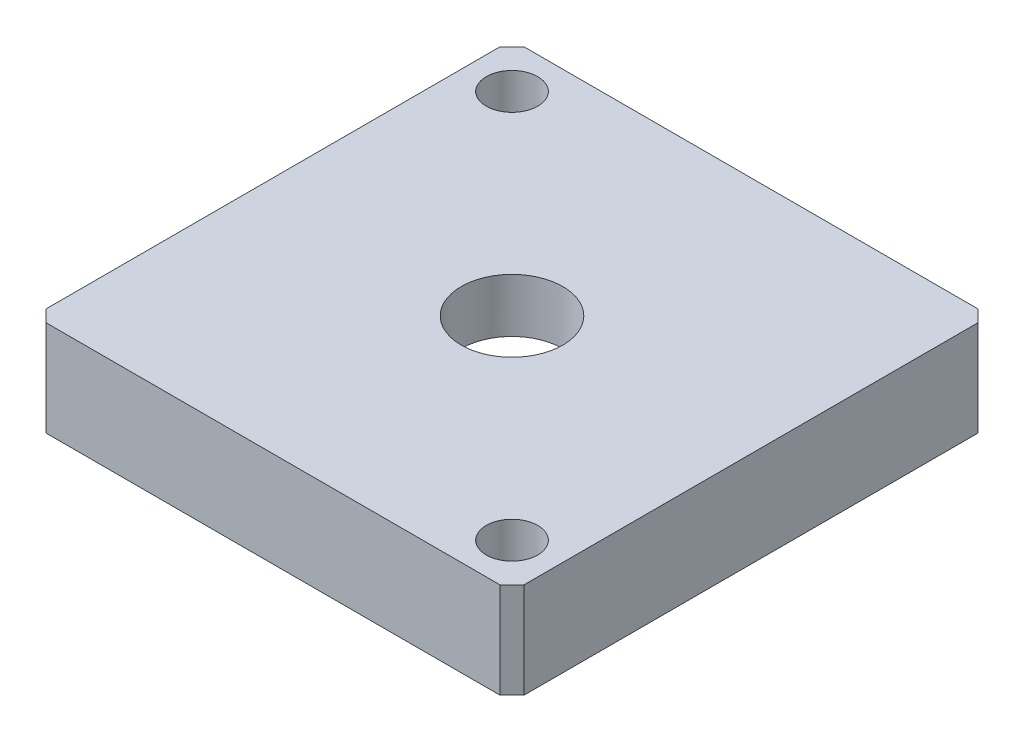
SolidWorks part; units mm, degrees
ref_plane "Front Plane" through (0, 0, 0) normal (0, 0, 1) x (1, 0, 0)
ref_plane "Top Plane" through (0, 0, 0) normal (0, 1, 0) x (1, 0, 0)
ref_plane "Right Plane" through (0, 0, 0) normal (1, 0, 0) x (0, 0, -1)
sketch "Sketch1" plane through (0, 0, 0) normal (0, 1, 0) x (1, 0, 0)
  line L1 (-20, 20) -> (20, 20)
  line L2 (-20, 20) -> (-20, -20)
  line L3 (-20, -20) -> (20, -20)
  line L4 (20, 20) -> (20, -20)
  line L5 (-20, 20) -> (20, -20) construction
  line L6 (-20, -20) -> (20, 20) construction
  point P0 (0, 0)
  dimension "D1" = 40
  dimension "D2" = 40
extrude "Boss-Extrude1" add sketch "Sketch1" along normal blind 8
chamfer "Chamfer1" distance 1 angle 45 4 edges at (-20, 4, 20) (20, 4, 20) (-20, 4, -20) (20, 4, -20)
sketch "Sketch2" plane through (0, 0, 0) normal (0, -1, 0) x (1, 0, 0)
  circle A0 centre (0, 0) radius 15.5
  dimension "D1" = 31
extrude "Cut-Extrude1" cut sketch "Sketch2" against normal blind 3.5
sketch "Sketch3" plane through (0, 8, 0) normal (0, 1, 0) x (1, 0, 0)
  circle A0 centre (0, 0) radius 4.25
  dimension "D1" = 8.5
extrude "Cut-Extrude2" cut sketch "Sketch3" against normal through all
sketch "Sketch4" plane through (0, 0, 0) normal (0, -1, 0) x (1, 0, 0)
  circle A0 centre (16.2635, 16.2635) radius 2.15
  circle A1 centre (-16.2635, -16.2635) radius 2.15
extrude "Cut-Extrude3" cut sketch "Sketch4" against normal blind 10
